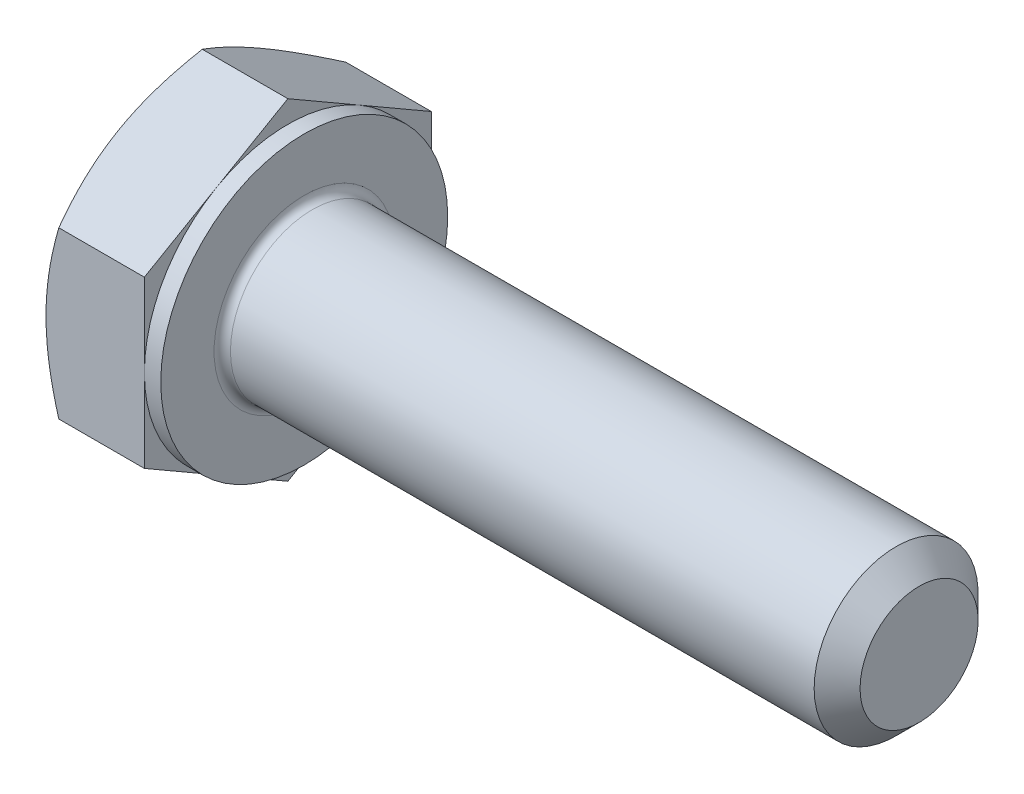
from build123d import *

# Parameters (mm, degrees)
EXTRUDE_358_DEPTH = 2.8
SKETCH_4_W        = 0.4
SKETCH_4_H        = 10.541451884
CHAMFER_1889_SIZE = 0.56
FILLET_1942_R     = 0.2


with BuildPart() as part:
    # 草图1 → Extrude 358 (new body)
    with BuildSketch(Plane(origin=(0, 0, 0), x_dir=(0, 0, -1), z_dir=(1, 0, 0))):
        Polygon((3.5, 2.020725942), (3.5, -2.020725942), (0, -4.041451884), (-3.5, -2.020725942), (-3.5, 2.020725942), (0, 4.041451884), align=None)
    extrude(amount=EXTRUDE_358_DEPTH)

    # 草图2 → 凸台-旋转1 (revolve)
    with BuildSketch(Plane.XY, mode=Mode.PRIVATE) as revolve_1_sk:
        Polygon((0, 0), (17.8, 0), (17.8, 1.3938), (17.8, 2), (0, 2), align=None)
    revolve(revolve_1_sk.sketch.rotate(Axis((0, 0, 0), (1, 0, 0)), 90), axis=Axis((0, 0, 0), (1, 0, 0)))

    # 草图3 → 切除-旋转1 (revolve, cut)
    with BuildSketch(Plane.XY):
        Polygon((0, 3.5), (3.199358737, 9.041451884), (3.199358737, 14.041451884), (-10, 14.041451884), (-10, 3.5), align=None)
    revolve(axis=Axis((0, 0, 0), (1, 0, 0)), mode=Mode.SUBTRACT)

    # 草图5 → 切除-旋转2 (revolve, cut)
    with BuildSketch(Plane.XY):
        Polygon((2.8, 3.5), (-0.399358737, 9.041451884), (-0.399358737, 14.041451884), (9.600641263, 14.041451884), (9.600641263, 3.5), align=None)
    revolve(axis=Axis((0, 0, 0), (1, 0, 0)), mode=Mode.SUBTRACT)

    # 草图4 → 切除-旋转3 (revolve, cut)
    with BuildSketch(Plane.XY, mode=Mode.PRIVATE) as cut_revolve_3_sk:
        with Locations((2.6, 8.770725942)):
            Rectangle(SKETCH_4_W, SKETCH_4_H)
    revolve(cut_revolve_3_sk.sketch.rotate(Axis((0, 0, 0), (1, 0, 0)), 270), axis=Axis((0, 0, 0), (1, 0, 0)), mode=Mode.SUBTRACT)

    # Chamfer 1889
    chamfer_1889_edges = [part.edges().sort_by_distance(p)[0] for p in [
        (17.8, 0, -2),
    ]]
    chamfer(chamfer_1889_edges, length=CHAMFER_1889_SIZE)

    # Fillet 1942
    fillet_1942_edges = [part.edges().sort_by_distance(p)[0] for p in [
        (2.8, 0, -2),
    ]]
    fillet(fillet_1942_edges, radius=FILLET_1942_R)


solid = part.part
